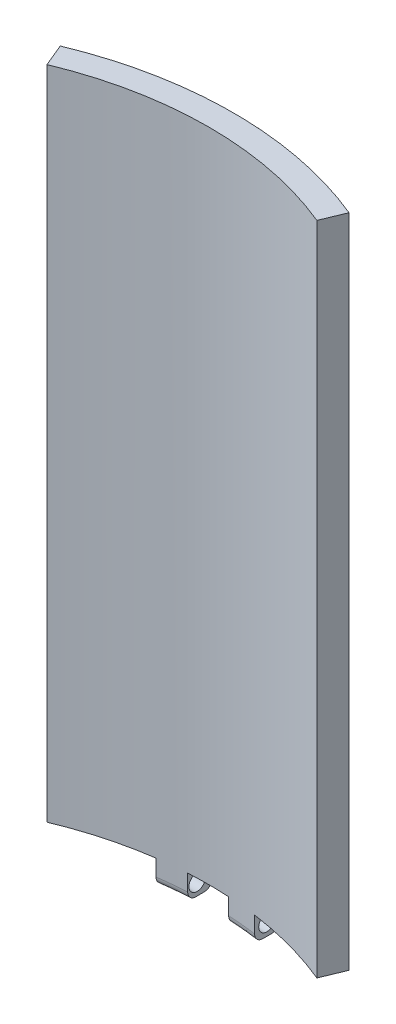
SolidWorks part; units mm, degrees
ref_plane "前视基准面" through (0, 0, 0) normal (0, 0, 1) x (1, 0, 0)
ref_plane "上视基准面" through (0, 0, 0) normal (0, 1, 0) x (1, 0, 0)
ref_plane "右视基准面" through (0, 0, 0) normal (1, 0, 0) x (0, 0, -1)
ref_plane "基准面4" through (0, 80, 0) normal (0, 1, 0) x (1, 0, 0)
sketch "草图3" plane through (0, 0, 0) normal (0, 1, 0) x (1, 0, 0)
  line L0 (0, 0) -> (0, 50000) construction
  line L1 (0, 0) -> (19134.1716, 46193.9766) construction
  line L2 (0, 0) -> (19134.1716, -46193.9766) construction
  line L3 (-17.6034, 42.4985) -> (-16.4554, 39.7268)
  line L4 (17.6034, 42.4985) -> (16.4554, 39.7268)
  arc A0 (-17.6034, 42.4985) -> (17.6034, 42.4985) centre (0, 0) cw
  arc A1 (-16.4554, 39.7268) -> (16.4554, 39.7268) centre (0, 0) cw
  dimension "D3" = 46
  dimension "D4" = 43
  dimension "D1" = 22.5
  dimension "D2" = 22.5
sketch "草图4" plane through (0, 80, 0) normal (0, 1, 0) x (1, 0, 0)
  line L0 (0, 0) -> (12940.9523, -48296.2913) construction
  line L1 (-17.6034, 42.4985) -> (-16.4554, 39.7268)
  line L2 (0, 0) -> (12940.9523, 48296.2913) construction
  line L3 (17.6034, 42.4985) -> (16.4554, 39.7268)
  line L4 (0, 0) -> (0, -50000) construction
  line L5 (0, 0) -> (19134.1716, -46193.9766) construction
  line L6 (0, 0) -> (19134.1716, 46193.9766) construction
  line L8 (0, -200000) -> (0, 250000) construction
  arc A0 (-16.4554, 39.7268) -> (16.4554, 39.7268) centre (0, 0) cw
  arc A1 (16.4554, 39.7268) -> (-16.4554, 39.7268) centre (0, 0) ccw construction
  arc A2 (-17.6034, 42.4985) -> (17.6034, 42.4985) centre (0, 0) cw
  arc A3 (17.6034, 42.4985) -> (-17.6034, 42.4985) centre (0, 0) ccw construction
  point P18 (-17.0294, 41.1126)
  dimension "D1" = 22.5
  dimension "D2" = 22.5
loft "放样1" add profiles "草图4", "草图3"
sketch "草图6" plane through (0, 0, 0) normal (0, -1, 0) x (1, 0, 0)
  line L1 (-6.0092, -42.9273) -> (-2.5, -42.9273)
  line L2 (-6.0092, -42.9273) -> (-6.0092, -45.6058)
  line L3 (-6.0092, -45.6058) -> (-2.5, -45.6058)
  line L4 (-2.5, -42.9273) -> (-2.5, -45.6058)
  line L9 (0, 200000) -> (0, -250000) construction
  line L10 (-6.0092, -42.9273) -> (-6.0092, -42.578)
  line L11 (-2.5, -45.6058) -> (-2.5, -45.932)
  line L12 (0, -43.9734) -> (0, -50043.9734) construction
  line L13 (2.5, -45.6058) -> (2.5, -45.932)
  line L14 (6.0092, -42.9273) -> (6.0092, -42.578)
  line L15 (2.5, -42.9273) -> (2.5, -45.6058)
  line L16 (6.0092, -45.6058) -> (2.5, -45.6058)
  line L17 (6.0092, -42.9273) -> (6.0092, -45.6058)
  line L18 (6.0092, -42.9273) -> (2.5, -42.9273)
  arc A0 (-17.6034, -42.4985) -> (17.6034, -42.4985) centre (0, 0) ccw construction
  arc A1 (-16.4554, -39.7268) -> (16.4554, -39.7268) centre (0, 0) ccw construction
  arc A2 (-6.0092, -42.578) -> (-2.5, -42.9273) centre (0, 0) ccw
  arc A3 (-6.0092, -45.6058) -> (-2.5, -45.932) centre (0, 0) ccw
  arc A4 (6.0092, -45.6058) -> (2.5, -45.932) centre (0, 0) cw
  arc A5 (6.0092, -42.578) -> (2.5, -42.9273) centre (0, 0) cw
  dimension "D1" = 2.5
extrude "凸台-拉伸1" add sketch "草图6" along normal blind 3
sketch "草图7" plane through (0, 0, 0) normal (1, 0, 0) x (0, 0, -1)
  circle A0 centre (44.0813, -1.5184) radius 1
  dimension "D1" = 2
extrude "切除-拉伸2" cut sketch "草图7" against normal mid plane 13
fillet "圆角3" radius 1 4 edges
sketch "草图8" plane through (0, 0, 0) normal (0, 0, 1) x (1, 0, 0)
  circle A0 centre (0, 40) radius 1.5
  dimension "D1" = 3
  dimension "D2" = 40
extrude "切除-拉伸3" cut sketch "草图8" against normal through all from offset 43.5
